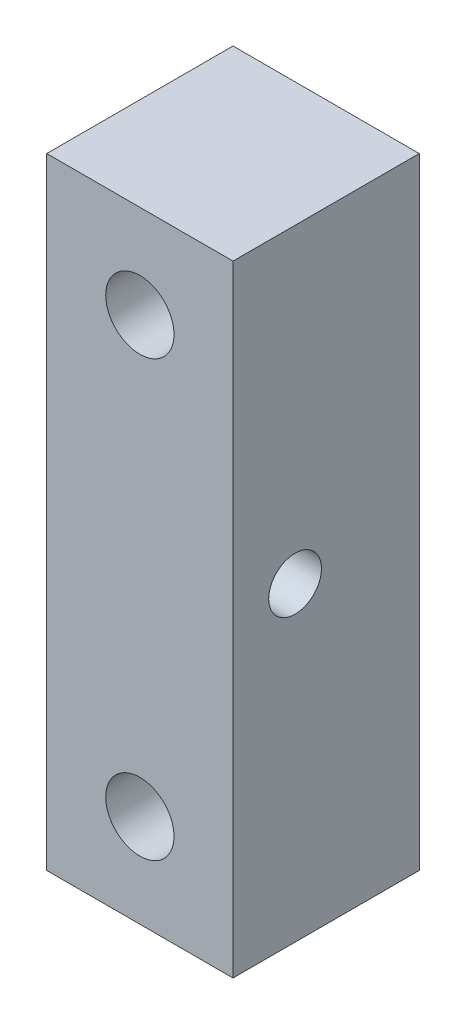
from build123d import *

# Parameters (mm, degrees)
SKETCH_1_W                = 30
SKETCH_1_H                = 30
EXTRUDE_1_DEPTH           = 100
HOLE_WIZARD_1_D           = 11
HOLE_WIZARD_1_CBORE_D     = 18
HOLE_WIZARD_1_CBORE_DEPTH = 11
HOLE_WIZARD_M10_1_D       = 8.5


with BuildPart() as part:
    # 草图1 → 凸台-拉伸1 (new body)
    with BuildSketch(Plane(origin=(0, 0, 0), x_dir=(1, 0, 0), z_dir=(0, 1, 0))):
        Rectangle(SKETCH_1_W, SKETCH_1_H)
    extrude(amount=EXTRUDE_1_DEPTH)

    # 打孔尺寸(%根据)内六角圆柱头螺钉的类型1 (through all)
    with Locations(Plane(origin=(0, 0, -15), x_dir=(-1, 0, 0), z_dir=(0, 0, -1))):
        with Locations((0, 15), (0, 85)):
            CounterBoreHole(HOLE_WIZARD_1_D / 2, HOLE_WIZARD_1_CBORE_D / 2, HOLE_WIZARD_1_CBORE_DEPTH)

    # M10 螺纹孔1 (through all)
    with Locations(Plane.ZY.offset(15)):
        with Locations((5, 50)):
            Hole(HOLE_WIZARD_M10_1_D / 2)


solid = part.part
